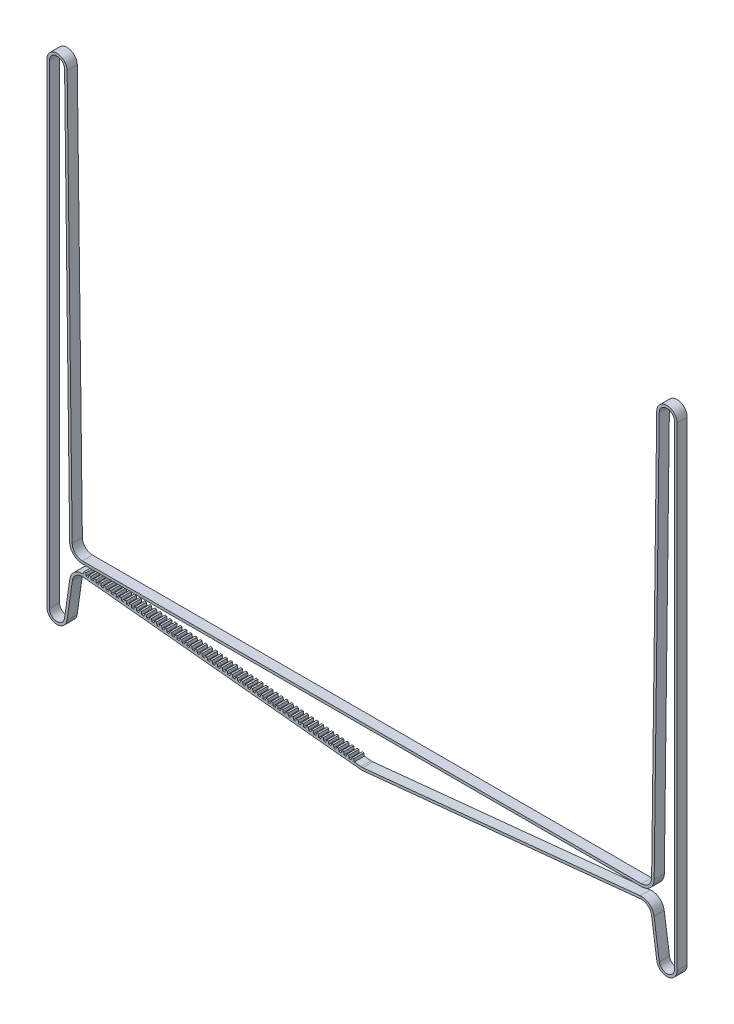
SolidWorks part; units mm, degrees
ref_plane "Front Plane" through (0, 0, 0) normal (0, 0, 1) x (1, 0, 0)
ref_plane "Top Plane" through (0, 0, 0) normal (0, 1, 0) x (1, 0, 0)
ref_plane "Right Plane" through (0, 0, 0) normal (1, 0, 0) x (0, 0, -1)
sketch "Sketch1" plane through (0, 0, 0) normal (0, 0, 1) x (1, 0, 0)
  line L0 (-136.6195, -129.3818) -> (27.0317, -145.8142)
  line L1 (27.781, -138.3518) -> (27.781, -162.8383) construction
  line L2 (192.1816, -129.3818) -> (28.5303, -145.8142)
  line L3 (-136.4697, -127.8893) -> (27.1816, -144.3218)
  line L4 (192.0317, -127.8893) -> (28.3805, -144.3218)
  line L16 (-158.219, 124.6482) -> (-158.219, -155.3518)
  line L17 (-146.2801, -156.2059) -> (-143.1579, -134.4976)
  line L19 (198.7199, -134.4976) -> (201.8421, -156.2059)
  line L20 (213.781, -155.3518) -> (213.781, 124.6482)
  line L21 (201.7815, 124.7232) -> (198.7805, -115.4267)
  line L22 (192.781, -121.3518) -> (-137.219, -121.3518)
  line L23 (-143.2185, -115.4267) -> (-146.2195, 124.7232)
  line L32 (203.2814, 124.7045) -> (200.2804, -115.4455)
  line L33 (212.281, -155.3518) -> (212.281, 124.6482)
  line L34 (200.2046, -134.2841) -> (203.3268, -155.9924)
  line L36 (-147.7648, -155.9924) -> (-144.6426, -134.2841)
  line L37 (-156.719, 124.6482) -> (-156.719, -155.3518)
  line L38 (-144.7184, -115.4455) -> (-147.7193, 124.7045)
  line L39 (192.781, -122.8518) -> (-137.219, -122.8518)
  arc A2 (-136.6195, -129.3818) -> (-143.1579, -134.4976) centre (-137.219, -135.3518) ccw
  arc A3 (27.0317, -145.8142) -> (28.5303, -145.8142) centre (27.781, -138.3518) ccw
  arc A4 (192.1816, -129.3818) -> (198.7199, -134.4976) centre (192.781, -135.3518) cw
  arc A5 (-136.4697, -127.8893) -> (-144.6426, -134.2841) centre (-137.219, -135.3518) ccw
  arc A6 (27.1816, -144.3218) -> (28.3805, -144.3218) centre (27.781, -138.3518) ccw
  arc A7 (192.0317, -127.8893) -> (200.2046, -134.2841) centre (192.781, -135.3518) cw
  arc A16 (-146.2195, 124.7232) -> (-158.219, 124.6482) centre (-152.219, 124.6482) ccw
  arc A17 (-158.219, -155.3518) -> (-146.2801, -156.2059) centre (-152.219, -155.3518) ccw
  arc A20 (201.8421, -156.2059) -> (213.781, -155.3518) centre (207.781, -155.3518) ccw
  arc A21 (213.781, 124.6482) -> (201.7815, 124.7232) centre (207.781, 124.6482) ccw
  arc A22 (192.781, -121.3518) -> (198.7805, -115.4267) centre (192.781, -115.3518) ccw
  arc A23 (-143.2185, -115.4267) -> (-137.219, -121.3518) centre (-137.219, -115.3518) ccw
  arc A32 (212.281, 124.6482) -> (203.2814, 124.7045) centre (207.781, 124.6482) ccw
  arc A33 (203.3268, -155.9924) -> (212.281, -155.3518) centre (207.781, -155.3518) ccw
  arc A36 (-156.719, -155.3518) -> (-147.7648, -155.9924) centre (-152.219, -155.3518) ccw
  arc A37 (-147.7193, 124.7045) -> (-156.719, 124.6482) centre (-152.219, 124.6482) ccw
  arc A38 (-144.7184, -115.4455) -> (-137.219, -122.8518) centre (-137.219, -115.3518) ccw
  arc A39 (192.781, -122.8518) -> (200.2804, -115.4455) centre (192.781, -115.3518) ccw
  dimension "D1" = 1.5
extrude "Boss-Extrude1" add sketch "Sketch1" along normal blind 6
sketch "Sketch2" plane through (0, 0, 6) normal (0, 0, 1) x (1, 0, 0)
  line L1 (-136.4697, -127.8893) -> (27.1816, -144.3218) construction
  line L2 (22.9549, -142.3898) -> (21.9599, -142.2899)
  line L3 (21.9599, -142.2899) -> (21.4101, -143.7422)
  line L4 (21.4101, -143.7422) -> (23.2049, -143.9225)
  line L5 (22.9549, -142.3898) -> (23.2049, -143.9225)
  dimension "D3" = 75
extrude "Boss-Extrude2" add sketch "Sketch2" against normal blind 6
pattern_linear "LPattern1" count 54 spacing 3 along (-0.995, 0.0999, 0) of "Boss-Extrude2"
